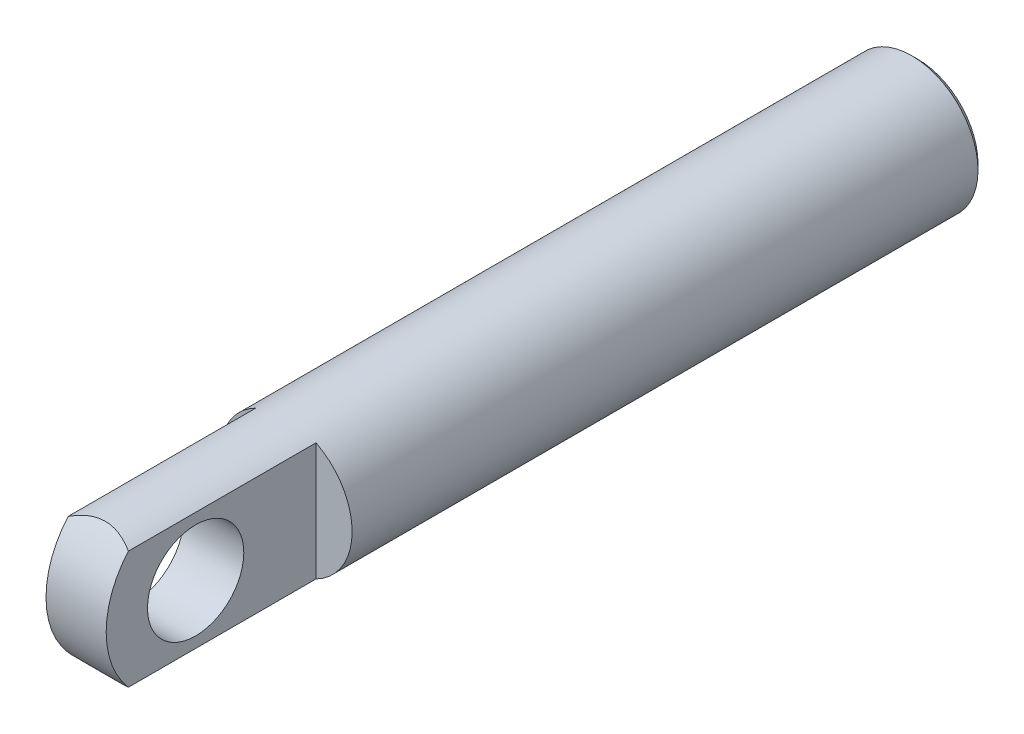
from build123d import *

# Parameters (mm, degrees)
SKETCH1_R                  = 11
BOSS_EXTRUDE1_DEPTH        = 140
CUT_EXTRUDE1_DEPTH         = 141.861634237
CUT_EXTRUDE1_DEPTH_BACK    = 35
SKETCH2_W                  = 16.868879615
SKETCH2_H                  = 32.554880476
SKETCH2_W_2                = 13.301543069
SKETCH2_H_2                = 32.07054439
M12X1_5_TAPPED_HOLE1_D     = 10.5
M12X1_5_TAPPED_HOLE1_DEPTH = 99.5
M12X1_5_TAPPED_HOLE1_TIP   = 3.15451825
CHAMFER1_SIZE              = 1
SKETCH5_R                  = 8
CUT_EXTRUDE2_DEPTH         = 142.340015565


with BuildPart() as part:
    # Sketch1 → Boss-Extrude1 (new body)
    with BuildSketch(Plane.XY):
        Circle(SKETCH1_R)
    extrude(amount=BOSS_EXTRUDE1_DEPTH)

    # Sketch2 → Cut-Extrude1 (cut, two sides: drawn at the far end of the back side and taken through both)
    with BuildSketch(Plane.XY.offset(140).offset(-CUT_EXTRUDE1_DEPTH_BACK)):
        with Locations((13.434439808, -1.928606663)):
            Rectangle(SKETCH2_W, SKETCH2_H)
        with Locations((-11.650771535, -1.34790253)):
            Rectangle(SKETCH2_W_2, SKETCH2_H_2)
    extrude(amount=CUT_EXTRUDE1_DEPTH + CUT_EXTRUDE1_DEPTH_BACK, mode=Mode.SUBTRACT)

    # M12x1.5 Tapped Hole1
    with Locations(Plane(origin=(-0.000266702, -0.000350185, 0), x_dir=(-1, 0, 0), z_dir=(0, 0, -1))):
        with Locations((0, 0)):
            Hole(M12X1_5_TAPPED_HOLE1_D / 2, depth=M12X1_5_TAPPED_HOLE1_DEPTH)
            with Locations((0, 0, -(M12X1_5_TAPPED_HOLE1_DEPTH + M12X1_5_TAPPED_HOLE1_TIP / 2))):  # 118° drill point
                Cone(0, M12X1_5_TAPPED_HOLE1_D / 2, M12X1_5_TAPPED_HOLE1_TIP, mode=Mode.SUBTRACT)

    # Chamfer1
    chamfer1_edges = [part.edges().sort_by_distance(p)[0] for p in [
        (-11, 0, 0),
    ]]
    chamfer(chamfer1_edges, length=CHAMFER1_SIZE)

    # Sketch5 → Cut-Extrude2 (cut, through all)
    with BuildSketch(Plane.ZY.offset(5)):
        with Locations(Location((125, 0, 0), (0, 0, 270))):
            Circle(SKETCH5_R)
        with BuildLine():
            Line((125, 14.866485564), (182.888016926, 36.743525749))
            Line((182.888016926, 36.743525749), (236.673487902, -7.349157171))
            Line((236.673487902, -7.349157171), (192.77085965, -51.061730756))
            Line((192.77085965, -51.061730756), (125, -14.866485564))
            ThreePointArc((125, -14.866485564), (139.866485564, 0), (125, 14.866485564))
        make_face()
    extrude(amount=-CUT_EXTRUDE2_DEPTH, mode=Mode.SUBTRACT)


solid = part.part
